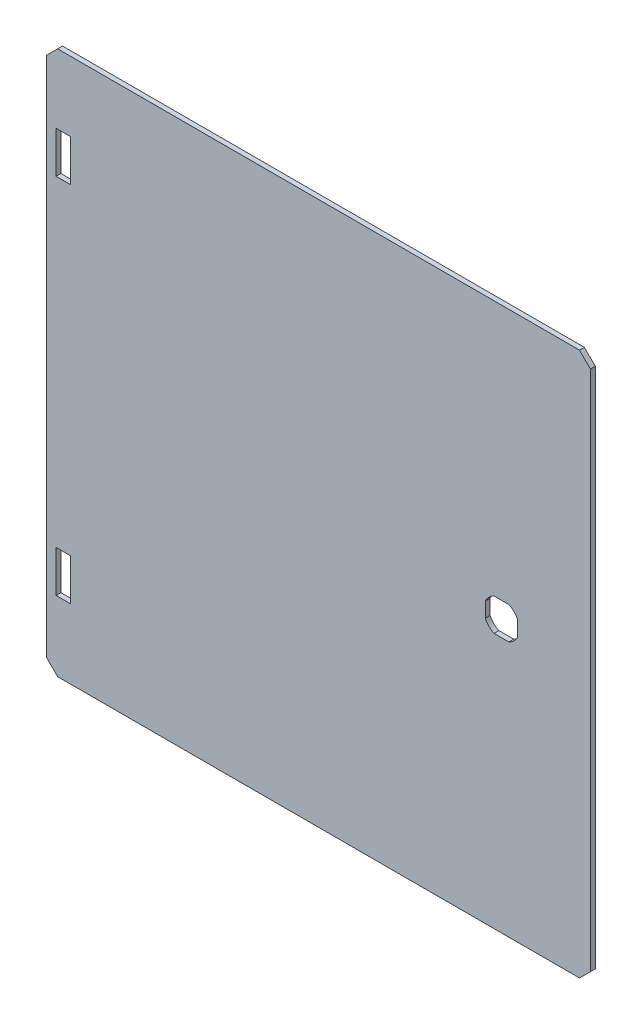
from build123d import *

# Parameters (mm, degrees)
SKETCH1_W           = 9
SKETCH1_H           = 25.7
BOSS_EXTRUDE1_DEPTH = 3
BOSS_EXTRUDE2_DEPTH = 3


with BuildPart() as part:
    # Sketch1 → Boss-Extrude1 (new body)
    with BuildSketch(Plane.XY):
        Polygon((165, -160), (165, 160), (160, 165), (-160, 165), (-165, 160), (-165, -160), (-160, -165), (160, -165), align=None)
        with BuildLine():
            Line((108.417424305, 10), (117.582575695, 10))
            ThreePointArc((117.582575695, 10), (120.778174593, 7.778174593), (123, 4.582575695))
            Line((123, 4.582575695), (123, -4.582575695))
            ThreePointArc((123, -4.582575695), (120.778174593, -7.778174593), (117.582575695, -10))
            Line((117.582575695, -10), (108.417424305, -10))
            ThreePointArc((108.417424305, -10), (105.221825407, -7.778174593), (103, -4.582575695))
            Line((103, -4.582575695), (103, 4.582575695))
            ThreePointArc((103, 4.582575695), (105.221825407, 7.778174593), (108.417424305, 10))
        make_face(mode=Mode.SUBTRACT)
        with Locations((-157.7, 112.15)):
            Rectangle(SKETCH1_W, SKETCH1_H, mode=Mode.SUBTRACT)
        with Locations((-157.7, -112.15)):
            Rectangle(SKETCH1_W, SKETCH1_H, mode=Mode.SUBTRACT)
    extrude(amount=BOSS_EXTRUDE1_DEPTH)

    # Sketch2 → Boss-Extrude2 (add)
    with BuildSketch(Plane.XY.offset(3)):
        Polygon((168, -161.242640687), (168, 161.242640687), (161.242640687, 168), (-161.242640687, 168), (-168, 161.242640687), (-168, -161.242640687), (-161.242640687, -168), (161.242640687, -168), align=None)
        Polygon((160, -165), (165, -160), (165, 160), (160, 165), (-160, 165), (-165, 160), (-165, -160), (-160, -165), align=None, mode=Mode.SUBTRACT)
    extrude(amount=-BOSS_EXTRUDE2_DEPTH)


solid = part.part
